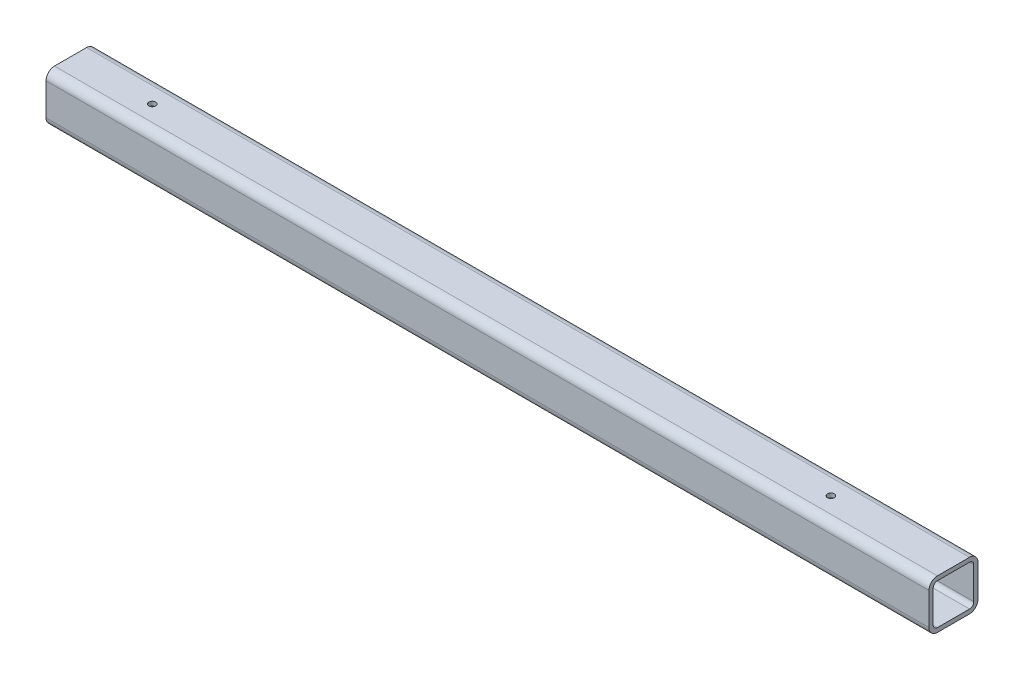
SolidWorks part; units mm, degrees
ref_plane "前视基准面" through (0, 0, 0) normal (0, 0, 1) x (1, 0, 0)
ref_plane "上视基准面" through (0, 0, 0) normal (0, 1, 0) x (1, 0, 0)
ref_plane "右视基准面" through (0, 0, 0) normal (1, 0, 0) x (0, 0, -1)
sketch3d "3D草图1"
  line L0 (0, 0, 0) -> (540, 0, 0)
  dimension "D1" = 540
other "结构构件1"
ref_plane "基准面1" through (0, 0, 0) normal (1, 0, 0) x (0, 0, -1)
sketch "Sketch1" plane through (0, 0, 0) normal (1, 0, 0) x (0, 0, -1)
  line L0 (-9.8, -12.4) -> (9.8, -12.4)
  line L1 (-12.4, -9.8) -> (-12.4, 9.8)
  line L2 (9.8, 12.4) -> (-9.8, 12.4)
  line L3 (12.4, 9.8) -> (12.4, -9.8)
  line L4 (-9.8, -15) -> (9.8, -15)
  line L5 (-15, -9.8) -> (-15, 9.8)
  line L6 (9.8, 15) -> (-9.8, 15)
  line L7 (15, 9.8) -> (15, -9.8)
  arc A0 (15, 9.8) -> (9.8, 15) centre (9.8, 9.8) ccw
  arc A1 (9.8, -15) -> (15, -9.8) centre (9.8, -9.8) ccw
  arc A2 (-15, -9.8) -> (-9.8, -15) centre (-9.8, -9.8) ccw
  arc A3 (-9.8, 15) -> (-15, 9.8) centre (-9.8, 9.8) ccw
  arc A4 (-9.8, 12.4) -> (-12.4, 9.8) centre (-9.8, 9.8) ccw
  arc A5 (12.4, 9.8) -> (9.8, 12.4) centre (9.8, 9.8) ccw
  arc A6 (9.8, -12.4) -> (12.4, -9.8) centre (9.8, -9.8) ccw
  arc A7 (-12.4, -9.8) -> (-9.8, -12.4) centre (-9.8, -9.8) ccw
  point P0 (-15, 0)
  point P1 (15, 0)
  point P2 (0, 15)
  point P3 (0, -15)
  point P4 (0, 0)
  point P5 (-15, -15)
  point P6 (15, -15)
  point P7 (15, 15)
  point P8 (-15, 15)
  point P33 (0, 0)
  dimension "D1" = 5.2
  dimension "Thickness" = 2.6
  dimension "V_leg" = 30
hole_wizard "M5 螺纹孔1" positions "草图2" profile "草图1" tap size "M5" standard "Iso" end condition through all
sketch "草图2" plane through (0, -15, 0) normal (0, -1, 0) x (-1, 0, 0)
  point P0 (-465, 0)
sketch "草图1" plane through (465, -15, 0) normal (1, 0, 0) x (0, 0, -1)
  line L0 (0, 0) -> (0, 30)
  line L1 (0, 30) -> (2.1, 30)
  line L2 (2.1, 30) -> (2.1, 0)
  line L5 (2.1, 0) -> (0, 0)
  line L11 (0, -6.35) -> (0, 107.95) construction
  dimension "通孔螺纹孔钻头直径" = 4.2
  dimension "通孔螺纹孔钻头深度" = 30
cosmetic thread "孔螺蚊线1" parameters "D2"=5
hole_wizard " 螺纹孔2" positions "草图4" profile "草图3" tap size "M5" standard "Iso" end condition through all
sketch "草图4" plane through (0, -15, 0) normal (0, -1, 0) x (-1, 0, 0)
  line L0 (0, 0) -> (-540, 0) construction
  line L1 (0, -9.8) -> (0, 9.8) construction
  point P0 (-50, 0)
  dimension "D1" = 50
cosmetic thread "孔螺蚊线2" parameters "D2"=5
sketch "草图3" plane through (50, -15, 0) normal (1, 0, 0) x (0, 0, -1)
  line L0 (0, 0) -> (0, 30)
  line L1 (0, 30) -> (2.1, 30)
  line L2 (2.1, 30) -> (2.1, 0)
  line L5 (2.1, 0) -> (0, 0)
  line L11 (0, -6.35) -> (0, 107.95) construction
  dimension "通孔螺纹孔钻头直径" = 4.2
  dimension "通孔螺纹孔钻头深度" = 30
